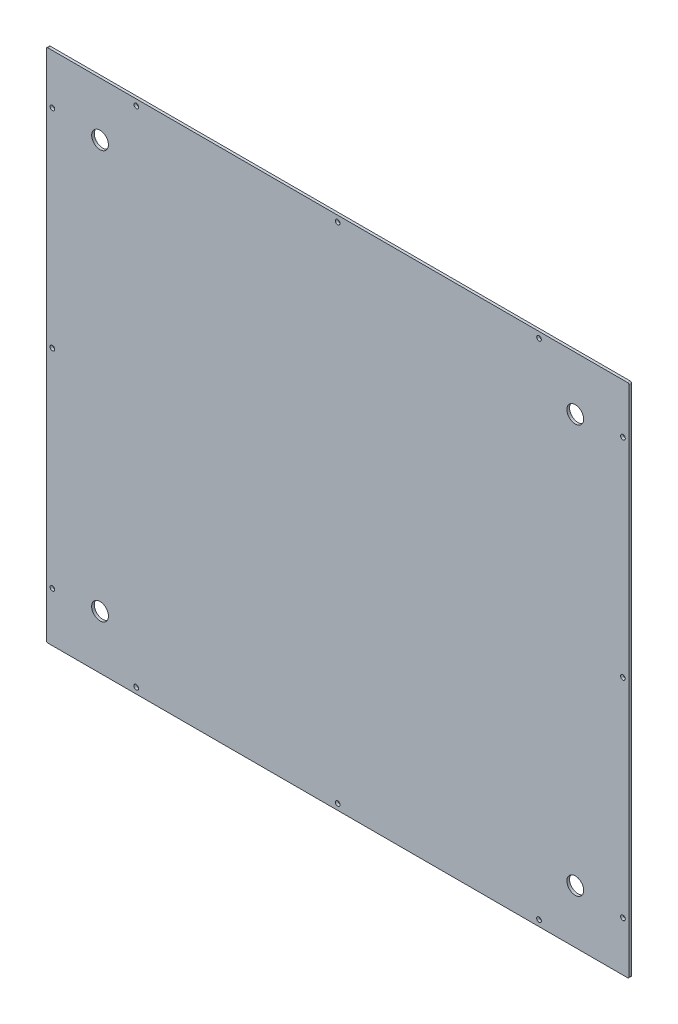
from build123d import *

# Parameters (mm, degrees)
SKETCH_1_W               = 868
SKETCH_1_H               = 768
EXTRUDE_1_DEPTH          = 4
FILLET_1_R               = 2
HOLE_WIZARD_M6_1_D       = 7
HOLE_WIZARD_M6_2_D       = 7
CUT_EXTRUDE_1_REACH      = 581.507
SKETCH_7_R               = 12.5
MIRROR_5_COPY_1_REACH    = 581.507
MIRROR_5_COPY_1_SKETCH_R = 12.5


with BuildPart() as part:
    # 草图1 → 凸台-拉伸1 (new body)
    with BuildSketch(Plane.XY):
        Rectangle(SKETCH_1_W, SKETCH_1_H)
    extrude(amount=EXTRUDE_1_DEPTH)

    # 圆角1
    fillet_1_edges = [part.edges().sort_by_distance(p)[0] for p in [
        (-434, 384, 2),
        (434, 384, 2),
        (434, -384, 2),
        (-434, -384, 2),
    ]]
    fillet(fillet_1_edges, radius=FILLET_1_R)

    # M6 间隙孔1 (through all)
    with Locations(Plane.XY.offset(4)):
        with Locations((-425, 310), (-425, -310), (-425, 0)):
            hole_wizard_m6_1 = Hole(HOLE_WIZARD_M6_1_D / 2)

    # 镜向2: M6 间隙孔1 across plane
    add(hole_wizard_m6_1.mirror(Plane(origin=(0, 0, 0), x_dir=(0, 0, 1), z_dir=(1, 0, 0))), mode=Mode.SUBTRACT)

    # M6 间隙孔2 (through all)
    with Locations(Plane.XY.offset(4)):
        with Locations((-300, 375), (300, 375), (0, 375)):
            hole_wizard_m6_2 = Hole(HOLE_WIZARD_M6_2_D / 2)

    # 镜向3: M6 间隙孔2 across plane
    add(hole_wizard_m6_2.mirror(Plane.ZX), mode=Mode.SUBTRACT)

    # 草图7 → 切除-拉伸1 (cut, up to next)
    with BuildSketch(Plane.XY.offset(4), mode=Mode.PRIVATE) as cut_extrude_1_sk1:
        with Locations((-354, -304)):
            Circle(SKETCH_7_R)
    cut_extrude_1_tool1 = extrude(cut_extrude_1_sk1.sketch, amount=-CUT_EXTRUDE_1_REACH, mode=Mode.PRIVATE) & part.part
    cut_extrude_1 = cut_extrude_1_tool1.solids().sort_by_distance((-354, -304, 4))[0]
    add(cut_extrude_1, mode=Mode.SUBTRACT)

    # 镜向4: 切除-拉伸1 across plane
    add(cut_extrude_1.mirror(Plane(origin=(0, 0, 0), x_dir=(0, 0, 1), z_dir=(1, 0, 0))), mode=Mode.SUBTRACT)

    # 镜向5: 切除-拉伸1 across plane
    add(cut_extrude_1.mirror(Plane.ZX), mode=Mode.SUBTRACT)

    # 镜向5 copy 1 sketch → 镜向5 copy 1 (cut, up to next)
    with BuildSketch(Plane(origin=(0, 0, 4), x_dir=(-1, 0, 0), z_dir=(0, 0, 1)), mode=Mode.PRIVATE) as mirror_5_copy_1_sk1:
        with Locations((-354, -304)):
            Circle(MIRROR_5_COPY_1_SKETCH_R)
    mirror_5_copy_1_tool1 = extrude(mirror_5_copy_1_sk1.sketch, amount=-MIRROR_5_COPY_1_REACH, mode=Mode.PRIVATE) & part.part
    add(mirror_5_copy_1_tool1.solids().sort_by_distance((354, 304, 4))[0], mode=Mode.SUBTRACT)


solid = part.part
